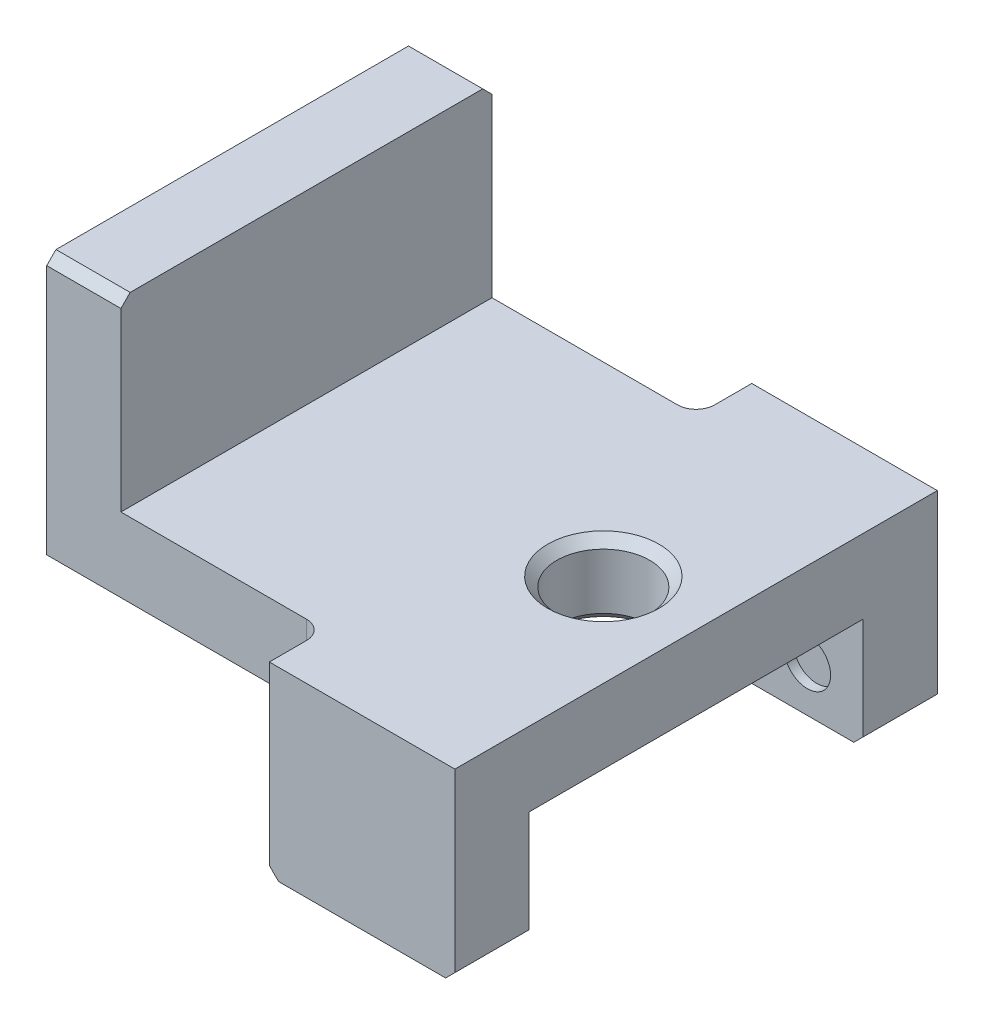
SolidWorks part; units mm, degrees
material "Q235-A"
ref_plane "Front Plane" through (0, 0, 0) normal (0, 0, 1) x (1, 0, 0)
ref_plane "Top Plane" through (0, 0, 0) normal (0, 1, 0) x (1, 0, 0)
ref_plane "Right Plane" through (0, 0, 0) normal (1, 0, 0) x (0, 0, -1)
sketch "Sketch1" plane through (0, 0, 0) normal (0, 1, 0) x (1, 0, 0)
  line L1 (0, 0) -> (50, 0)
  line L2 (0, 0) -> (0, -40)
  line L3 (0, -40) -> (50, -40)
  line L4 (50, 0) -> (50, -40)
  dimension "D1" = 50
  dimension "D2" = 40
extrude "Boss-Extrude1" add sketch "Sketch1" along normal blind 8
sketch "Sketch3" plane through (0, 8, 0) normal (0, 1, 0) x (1, 0, 0)
  line L0 (50, -40) -> (50, 0) construction
  line L1 (30, 6) -> (50, 6)
  line L2 (30, 6) -> (30, -46)
  line L3 (30, -46) -> (50, -46)
  line L4 (50, 6) -> (50, -46)
  line L5 (50, 0) -> (0, 0) construction
  line L6 (0, -40) -> (50, -40) construction
  dimension "D1" = 0
  dimension "D2" = 20
  dimension "D3" = 6
  dimension "D4" = 6
extrude "Boss-Extrude2" add sketch "Sketch3" against normal up to surface (8 mm away) up to face at (25, 0, 20)
sketch "Sketch2" plane through (0, 0, 0) normal (0, -1, 0) x (1, 0, 0)
  line L2 (40, 20) -> (50, 20) construction
  line L3 (50, 46) -> (50, -6) construction
  circle A0 centre (40, 20) radius 5
  dimension "D1" = 10
  dimension "D2" = 10
extrude "Cut-Extrude1" cut sketch "Sketch2" against normal through all
chamfer "Chamfer2" distance 1 angle 45 2 edges at (40, 8, 15) (40, 0, 15)
sketch "Sketch4" plane through (0, 0, 0) normal (0, 1, 0) x (1, 0, 0)
  line L0 (50, -46) -> (50, 6) construction
  line L1 (30, -46) -> (50, -46)
  line L2 (30, -46) -> (30, -38)
  line L3 (30, -38) -> (50, -38)
  line L4 (50, -46) -> (50, -38)
  line L6 (30, 6) -> (50, 6)
  line L7 (30, 6) -> (30, -2)
  line L8 (30, -2) -> (50, -2)
  line L9 (50, 6) -> (50, -2)
  dimension "D1" = 8
  dimension "D2" = 8
extrude "Boss-Extrude3" add sketch "Sketch4" against normal blind 12
chamfer "Chamfer4" distance 1 angle 45 4 edges at (50, -12, 42) (30, -12, 42) (50, -12, -2) (30, -12, -2)
fillet "Fillet1" radius 2 2 edges at (30, 4, 40) (30, 4, 0)
sketch "Sketch5" plane through (0, 8, 0) normal (0, 1, 0) x (1, 0, 0)
  line L0 (0, -40) -> (28, -40) construction
  line L1 (0, 0) -> (8, 0)
  line L2 (0, 0) -> (0, -40)
  line L3 (0, -40) -> (8, -40)
  line L4 (8, 0) -> (8, -40)
  dimension "D1" = 8
extrude "Boss-Extrude4" add sketch "Sketch5" along normal blind 20
chamfer "Chamfer5" distance 1 angle 45 2 edges at (4, 28, 0) (4, 28, 40)
sketch "Sketch6" plane through (0, 0, 2) normal (0, 0, 1) x (1, 0, 0)
  line L0 (31, -12) -> (49, -12) construction
  line L1 (50, -11) -> (50, 8) construction
  circle A0 centre (44, -7) radius 2.5
  circle A1 centre (36, -7) radius 2.5
  dimension "D1" = 5
  dimension "D2" = 8
  dimension "D3" = 6
extrude "Cut-Extrude2" cut sketch "Sketch6" against normal blind 1
sketch "Sketch7" plane through (0, 0, 38) normal (0, 0, -1) x (-1, 0, 0)
  circle A1 centre (-36, -7) radius 2.5
  circle A2 centre (-36, -7) radius 2.5
  circle A3 centre (-44, -7) radius 2.5
  circle A4 centre (-44, -7) radius 2.5
  dimension "D1" = 0
  dimension "D2" = 0
extrude "Cut-Extrude3" cut sketch "Sketch7" against normal blind 1
